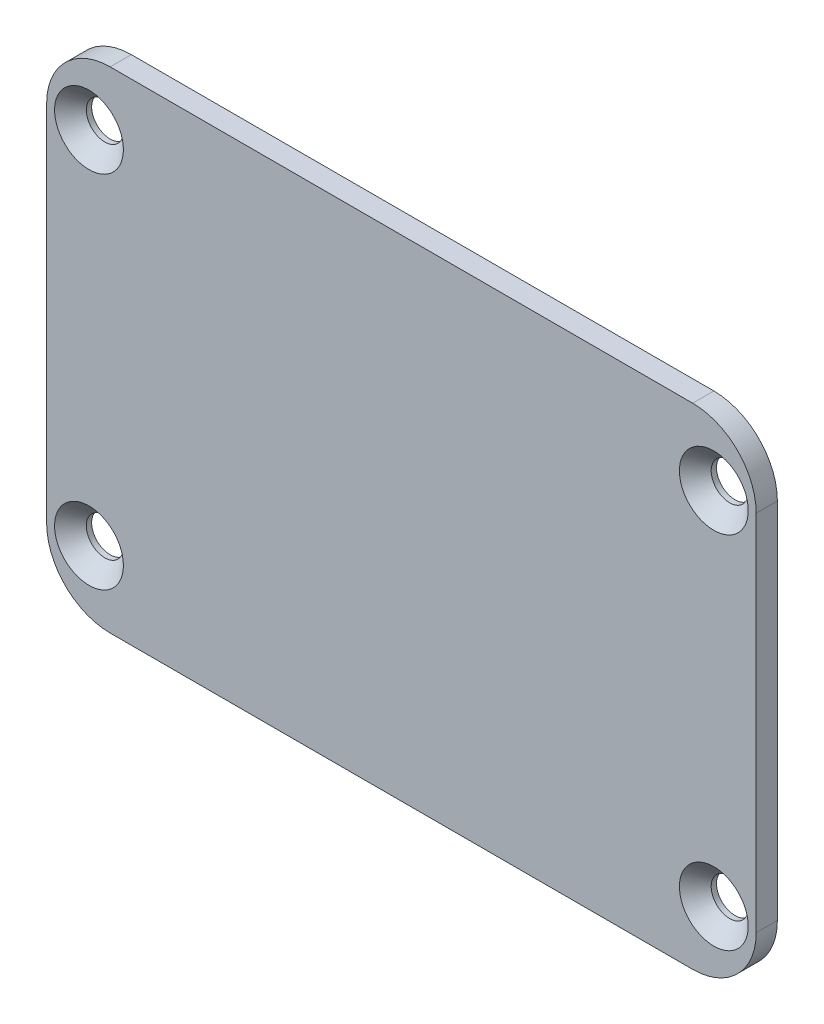
from build123d import *

# Parameters (mm, degrees)
SKETCH_1_W                  = 67
SKETCH_1_H                  = 46.3
EXTRUDE_1_DEPTH             = 2
FILLET_1_R                  = 6
HOLE_WIZARD_1_D             = 3.5
HOLE_WIZARD_1_DEPTH         = 10
HOLE_WIZARD_1_CSINK_D       = 6.5
HOLE_WIZARD_1_CSINK_ANGLE   = 90
PATTERN_LINEAR_1_COUNT      = 2
PATTERN_LINEAR_1_PITCH      = 34
PATTERN_LINEAR_1_COUNT_DIR2 = 2
PATTERN_LINEAR_1_PITCH_DIR2 = 59


with BuildPart() as part:
    # 草图1 → 拉伸1 (new body)
    with BuildSketch(Plane.XY):
        Rectangle(SKETCH_1_W, SKETCH_1_H)
    extrude(amount=EXTRUDE_1_DEPTH)

    # 圆角1
    fillet_1_edges = [part.edges().sort_by_distance(p)[0] for p in [
        (-33.5, 23.15, 1),
        (33.5, 23.15, 1),
        (33.5, -23.15, 1),
        (-33.5, -23.15, 1),
    ]]
    fillet(fillet_1_edges, radius=FILLET_1_R)

    # 孔1
    with Locations(Plane(origin=(-29.5, -17, 2), x_dir=(1, 0, 0), z_dir=(0, 0, 1))):
        with Locations((0, 0)):
            hole_wizard_1 = CounterSinkHole(HOLE_WIZARD_1_D / 2, HOLE_WIZARD_1_CSINK_D / 2, depth=HOLE_WIZARD_1_DEPTH, counter_sink_angle=HOLE_WIZARD_1_CSINK_ANGLE)

    # 阵列(线性)1: Hole Wizard 1 2 × 2
    with Locations(*[(j * PATTERN_LINEAR_1_PITCH_DIR2, i * PATTERN_LINEAR_1_PITCH, 0) for i in range(PATTERN_LINEAR_1_COUNT) for j in range(PATTERN_LINEAR_1_COUNT_DIR2) if (i, j) != (0, 0)]):
        add(hole_wizard_1, mode=Mode.SUBTRACT)


solid = part.part
